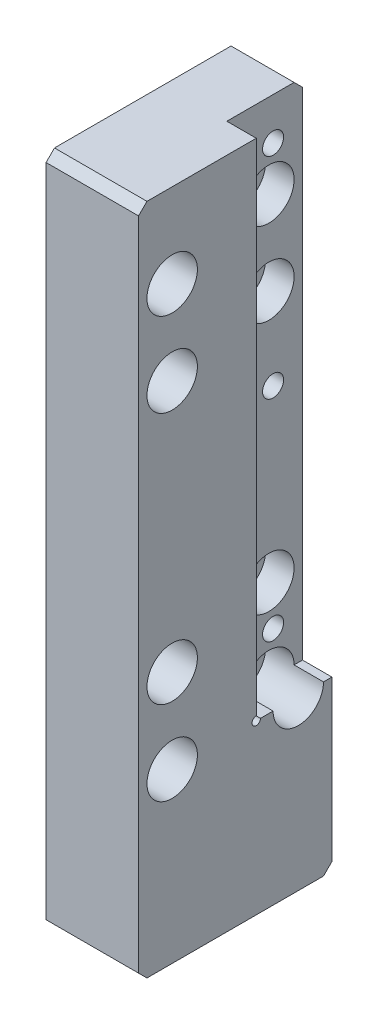
from build123d import *

# Parameters (mm, degrees)
SKETCH_1_W                = 11
SKETCH_1_H                = 23
EXTRUDE_1_DEPTH           = 80
CUT_EXTRUDE_1_DEPTH       = 3.5
HOLE_WIZARD_2_D           = 3.4
HOLE_WIZARD_2_CBORE_D     = 6
HOLE_WIZARD_2_CBORE_DEPTH = 6.9
HOLE_WIZARD_M5_1_D        = 4.2
HOLE_WIZARD_M5_1_DEPTH    = 12.4
HOLE_WIZARD_M5_1_TIP      = 1.2618073
HOLE_WIZARD_M3_1_D        = 2.5
CHAMFER_1_SIZE            = 1


with BuildPart() as part:
    # 草图1 → 凸台-拉伸1 (new body)
    with BuildSketch(Plane(origin=(0, 0, 0), x_dir=(1, 0, 0), z_dir=(0, 1, 0))):
        with Locations((5.5, 11.5)):
            Rectangle(SKETCH_1_W, SKETCH_1_H)
    extrude(amount=EXTRUDE_1_DEPTH)

    # 草图2 → 切除-拉伸1 (cut)
    with BuildSketch(Plane(origin=(11, 0, 0), x_dir=(0, 0, -1), z_dir=(1, 0, 0))):
        with BuildLine():
            Line((23, 80), (14, 80))
            Line((14, 80), (14, 20.5))
            ThreePointArc((14, 20.5), (13.646446609, 19.646446609), (14.5, 20))
            Line((14.5, 20), (23, 20))
            Line((23, 20), (23, 80))
        make_face()
    extrude(amount=-CUT_EXTRUDE_1_DEPTH, mode=Mode.SUBTRACT)

    # 打孔尺寸(%根据)内六角圆柱头螺钉的类型2 (through all)
    with Locations(Plane(origin=(11, 0, 0), x_dir=(0, 0, -1), z_dir=(1, 0, 0))):
        with Locations((4, 20), (4, 30), (19, 30), (19, 20), (4, 60), (4, 70), (19, 60), (19, 70)):
            CounterBoreHole(HOLE_WIZARD_2_D / 2, HOLE_WIZARD_2_CBORE_D / 2, HOLE_WIZARD_2_CBORE_DEPTH)

    # M5 螺纹孔1
    with Locations(Plane(origin=(0, 0, 0), x_dir=(-1, 0, 0), z_dir=(0, -1, 0))):
        with Locations((-5.5, 11.5)):
            Hole(HOLE_WIZARD_M5_1_D / 2, depth=HOLE_WIZARD_M5_1_DEPTH)
            with Locations((0, 0, -(HOLE_WIZARD_M5_1_DEPTH + HOLE_WIZARD_M5_1_TIP / 2))):  # 118° drill point
                Cone(0, HOLE_WIZARD_M5_1_D / 2, HOLE_WIZARD_M5_1_TIP, mode=Mode.SUBTRACT)

    # M3 螺纹孔1 (through all)
    with Locations(Plane(origin=(7.5, 0, 0), x_dir=(0, 0, -1), z_dir=(1, 0, 0))):
        with Locations((19.5, 25), (19.5, 50), (19.5, 75)):
            Hole(HOLE_WIZARD_M3_1_D / 2)

    # 倒角1
    chamfer_1_edges = [part.edges().sort_by_distance(p)[0] for p in [
        (3.75, 80, -23),
        (5.5, 80, 0),
        (5.5, 0, -23),
        (5.5, 0, 0),
    ]]
    chamfer(chamfer_1_edges, length=CHAMFER_1_SIZE)


solid = part.part
